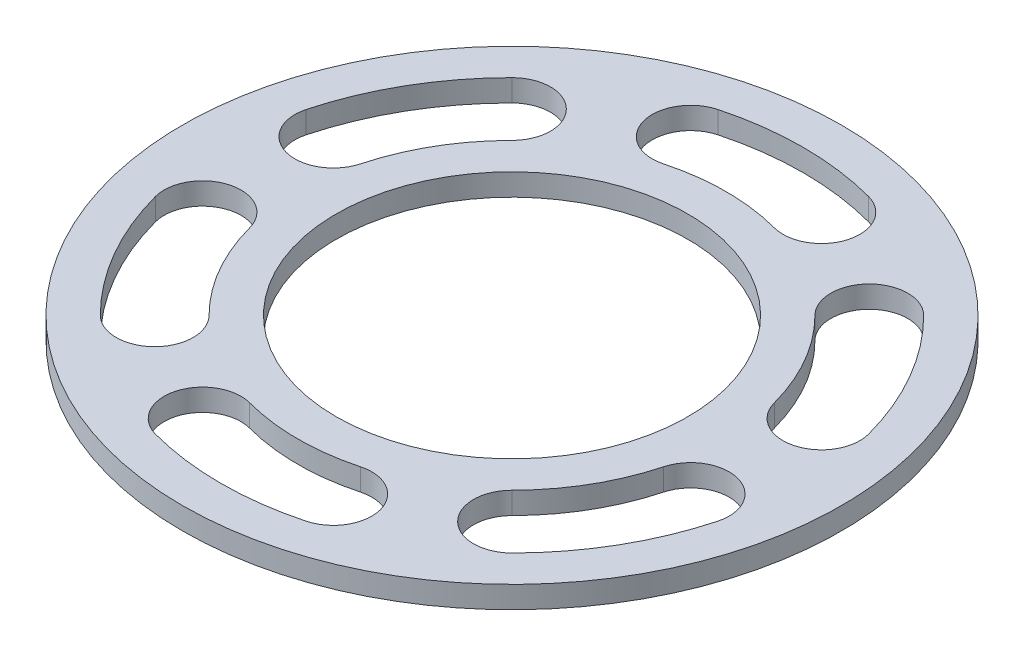
from build123d import *

# Parameters (mm, degrees)
SKETCH_1_R               = 30
SKETCH_1_R_2             = 16
EXTRUDE_1_DEPTH          = 2
CUT_EXTRUDE_1_DEPTH      = 43.473521163
CUT_EXTRUDE_1_DEPTH_BACK = 43.473521163


with BuildPart() as part:
    # 草图1 → 凸台-拉伸1 (new body)
    with BuildSketch(Plane(origin=(0, 0, 0), x_dir=(1, 0, 0), z_dir=(0, 1, 0))):
        with Locations(Location((0, 0, 0), (0, 0, 270))):
            Circle(SKETCH_1_R)
        with Locations(Location((0, 0, 0), (0, 0, 270))):
            Circle(SKETCH_1_R_2, mode=Mode.SUBTRACT)
    extrude(amount=EXTRUDE_1_DEPTH)

    # 草图2 → 切除-拉伸1 (cut, two sides: drawn at the far end of the back side and taken through both)
    with BuildSketch(Plane(origin=(0, 2, 0), x_dir=(1, 0, 0), z_dir=(0, 1, 0)).offset(-CUT_EXTRUDE_1_DEPTH_BACK)):
        with BuildLine():
            ThreePointArc((6.858704695, 25.597034397), (0, 26.5), (-6.858704695, 25.597034397))
            ThreePointArc((-6.858704695, 25.597034397), (-9.333578429, 21.310427347), (-5.046971379, 18.835553613))
            ThreePointArc((-5.046971379, 18.835553613), (0, 19.5), (5.046971379, 18.835553613))
            ThreePointArc((5.046971379, 18.835553613), (9.333578429, 21.310427347), (6.858704695, 25.597034397))
        make_face()
        with BuildLine():
            ThreePointArc((25.597034397, 6.858704695), (22.9496732, 13.25), (18.738329701, 18.738329701))
            ThreePointArc((18.738329701, 18.738329701), (13.788582233, 18.738329701), (13.788582233, 13.788582233))
            ThreePointArc((13.788582233, 13.788582233), (16.887495374, 9.75), (18.835553613, 5.046971379))
            ThreePointArc((18.835553613, 5.046971379), (23.122160663, 2.572097645), (25.597034397, 6.858704695))
        make_face()
        with BuildLine():
            ThreePointArc((18.738329701, -18.738329701), (22.9496732, -13.25), (25.597034397, -6.858704695))
            ThreePointArc((25.597034397, -6.858704695), (23.122160663, -2.572097645), (18.835553613, -5.046971379))
            ThreePointArc((18.835553613, -5.046971379), (16.887495374, -9.75), (13.788582233, -13.788582233))
            ThreePointArc((13.788582233, -13.788582233), (13.788582233, -18.738329701), (18.738329701, -18.738329701))
        make_face()
        with BuildLine():
            ThreePointArc((-6.858704695, -25.597034397), (0, -26.5), (6.858704695, -25.597034397))
            ThreePointArc((6.858704695, -25.597034397), (9.333578429, -21.310427347), (5.046971379, -18.835553613))
            ThreePointArc((5.046971379, -18.835553613), (0, -19.5), (-5.046971379, -18.835553613))
            ThreePointArc((-5.046971379, -18.835553613), (-9.333578429, -21.310427347), (-6.858704695, -25.597034397))
        make_face()
        with BuildLine():
            ThreePointArc((-25.597034397, -6.858704695), (-22.9496732, -13.25), (-18.738329701, -18.738329701))
            ThreePointArc((-18.738329701, -18.738329701), (-13.788582233, -18.738329701), (-13.788582233, -13.788582233))
            ThreePointArc((-13.788582233, -13.788582233), (-16.887495374, -9.75), (-18.835553613, -5.046971379))
            ThreePointArc((-18.835553613, -5.046971379), (-23.122160663, -2.572097645), (-25.597034397, -6.858704695))
        make_face()
        with BuildLine():
            ThreePointArc((-18.738329701, 18.738329701), (-22.9496732, 13.25), (-25.597034397, 6.858704695))
            ThreePointArc((-25.597034397, 6.858704695), (-23.122160663, 2.572097645), (-18.835553613, 5.046971379))
            ThreePointArc((-18.835553613, 5.046971379), (-16.887495374, 9.75), (-13.788582233, 13.788582233))
            ThreePointArc((-13.788582233, 13.788582233), (-13.788582233, 18.738329701), (-18.738329701, 18.738329701))
        make_face()
    extrude(amount=CUT_EXTRUDE_1_DEPTH + CUT_EXTRUDE_1_DEPTH_BACK, mode=Mode.SUBTRACT)


solid = part.part
